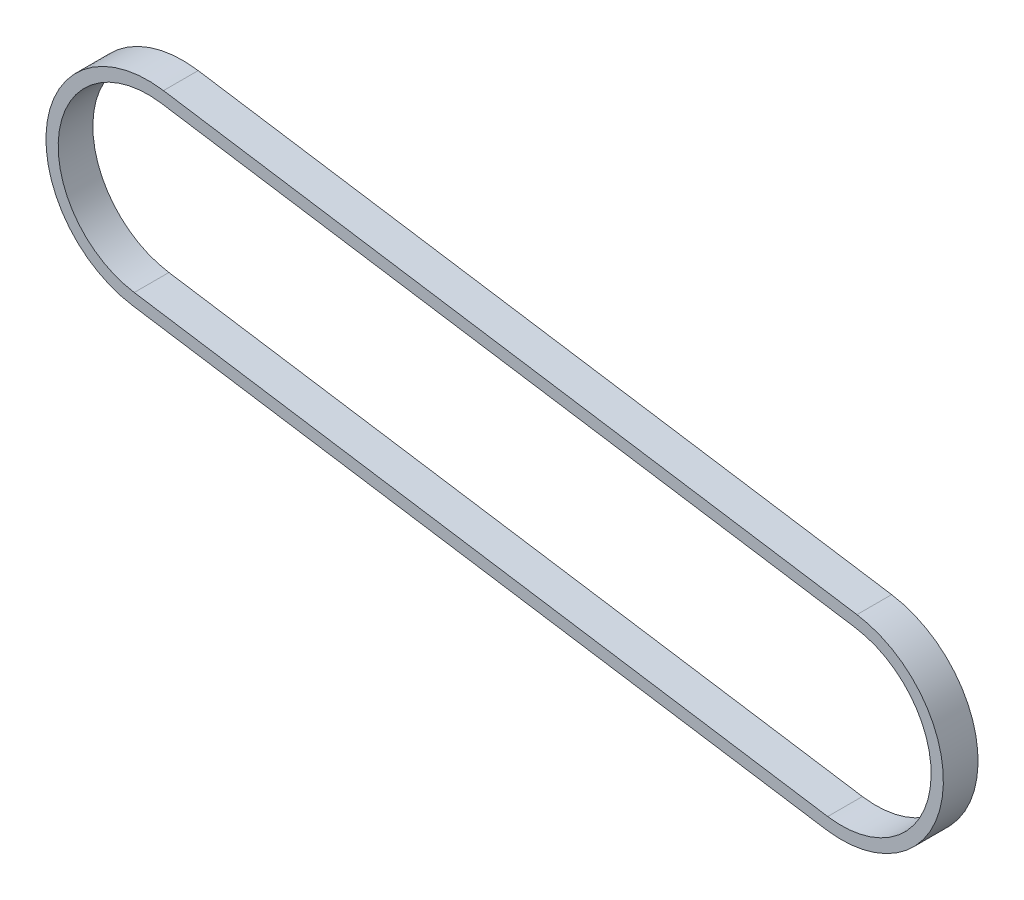
from build123d import *

# Parameters (mm, degrees)
EXTRUDE_THIN1_DEPTH = 8.5


with BuildPart() as part:
    # Sketch2 → Extrude-Thin1 (new, symmetric)
    with BuildSketch(Plane.XY):
        with BuildLine():
            Line((332.369838866, -101.914376866), (-7.630161134, -49.414376866))
            ThreePointArc((-7.630161134, -49.414376866), (-49.414376866, 7.630161134), (7.630161134, 49.414376866))
            Line((7.630161134, 49.414376866), (347.630161134, -3.085623134))
            ThreePointArc((347.630161134, -3.085623134), (389.414376866, -60.130161134), (332.369838866, -101.914376866))
        make_face()
        with BuildLine():
            Line((333.285458202, -95.984651642), (-6.714541798, -43.484651642))
            ThreePointArc((-6.714541798, -43.484651642), (-43.484651642, 6.714541798), (6.714541798, 43.484651642))
            Line((6.714541798, 43.484651642), (346.714541798, -9.015348358))
            ThreePointArc((346.714541798, -9.015348358), (383.484651642, -59.214541798), (333.285458202, -95.984651642))
        make_face(mode=Mode.SUBTRACT)
    extrude(amount=EXTRUDE_THIN1_DEPTH, both=True)


solid = part.part
